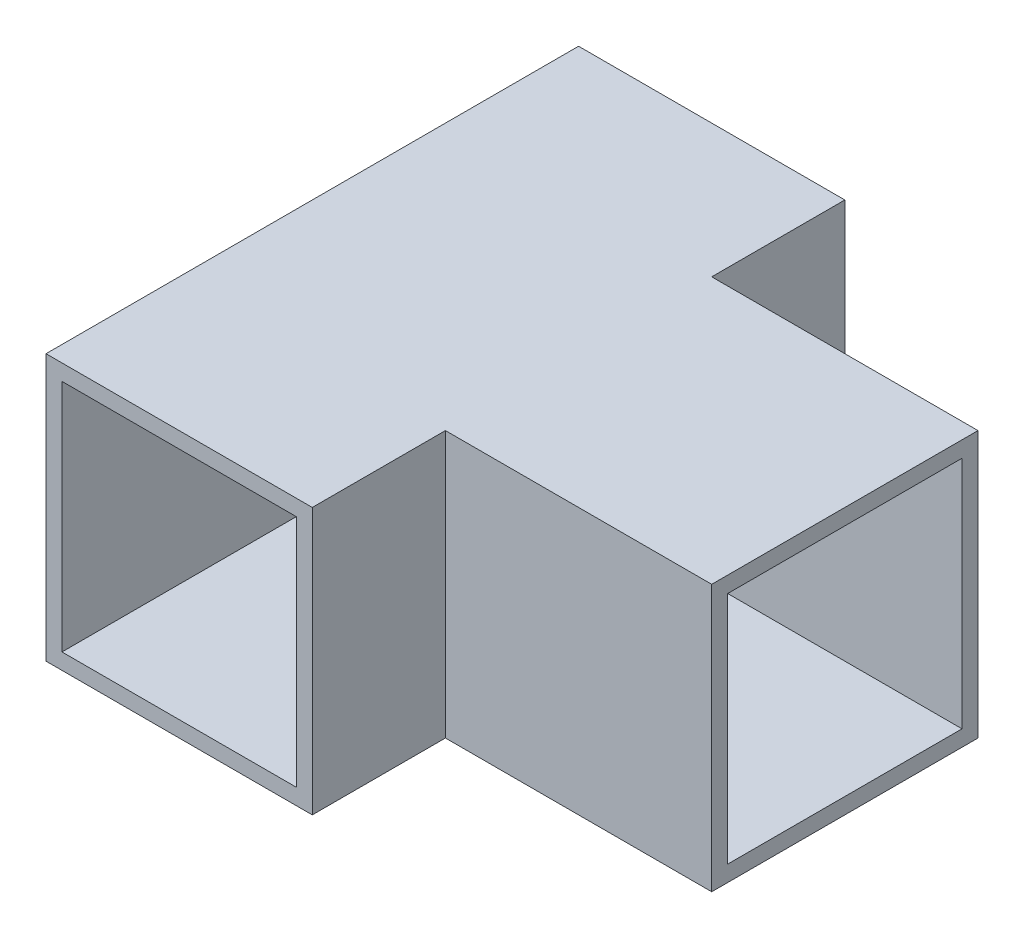
SolidWorks part; units mm, degrees
ref_plane "前视基准面" through (0, 0, 0) normal (0, 0, 1) x (1, 0, 0)
ref_plane "上视基准面" through (0, 0, 0) normal (0, 1, 0) x (1, 0, 0)
ref_plane "右视基准面" through (0, 0, 0) normal (1, 0, 0) x (0, 0, -1)
sketch "草图1" plane through (0, 0, 0) normal (0, 0, 1) x (1, 0, 0)
  line L0 (0, 0) -> (0, 50)
  line L1 (0, 50) -> (50, 50)
  line L2 (50, 50) -> (50, 0)
  line L3 (50, 0) -> (0, 0)
  line L4 (3, 3) -> (3, 47)
  line L5 (3, 47) -> (47, 47)
  line L6 (47, 47) -> (47, 3)
  line L7 (47, 3) -> (3, 3)
  dimension "D1" = 3
extrude "凸台-拉伸1" add sketch "草图1" along normal blind 200
sketch "草图2" plane through (0, 0, 200) normal (0, 0, 1) x (1, 0, 0)
  line L8 (-3, -3) -> (53, -3)
  line L9 (53, -3) -> (53, 53)
  line L10 (53, 53) -> (-3, 53)
  line L11 (-3, 53) -> (-3, -3)
  line L12 (-3, -3) -> (53, -3)
  line L13 (53, -3) -> (53, 53)
  line L14 (53, 53) -> (-3, 53)
  line L15 (-3, 53) -> (-3, -3)
  dimension "D1" = 3
extrude "切除-拉伸1" cut sketch "草图2" against normal blind 100
sketch "草图3" plane through (0, 0, 0) normal (-1, 0, 0) x (0, 0, 1)
  line L0 (50, 50) -> (25, 50)
  line L1 (100, 50) -> (0, 50) construction
  line L2 (50, 50) -> (75, 50)
  line L3 (50, 47) -> (28, 47)
  line L4 (28, 3) -> (28, 47)
  line L5 (75, 50) -> (75, 0)
  line L6 (100, 0) -> (0, 0) construction
  line L7 (75, 0) -> (25, 0)
  line L8 (25, 0) -> (25, 50)
  line L9 (72, 3) -> (28, 3)
  line L10 (72, 47) -> (72, 3)
  line L11 (50, 47) -> (72, 47)
  dimension "D1" = 3
extrude "凸台-拉伸3" add sketch "草图3" against normal blind 100
sketch "草图4" plane through (0, 0, 0) normal (0, 0, -1) x (-1, 0, 0)
  line L8 (-47, 3) -> (-3, 3)
  line L9 (-3, 3) -> (-3, 47)
  line L10 (-3, 47) -> (-47, 47)
  line L11 (-47, 47) -> (-47, 3)
  line L12 (-47, 3) -> (-3, 3)
  line L13 (-3, 3) -> (-3, 47)
  line L14 (-3, 47) -> (-47, 47)
  line L15 (-47, 47) -> (-47, 3)
  dimension "D1" = 3
extrude "切除-拉伸2" cut sketch "草图4" against normal blind 100
